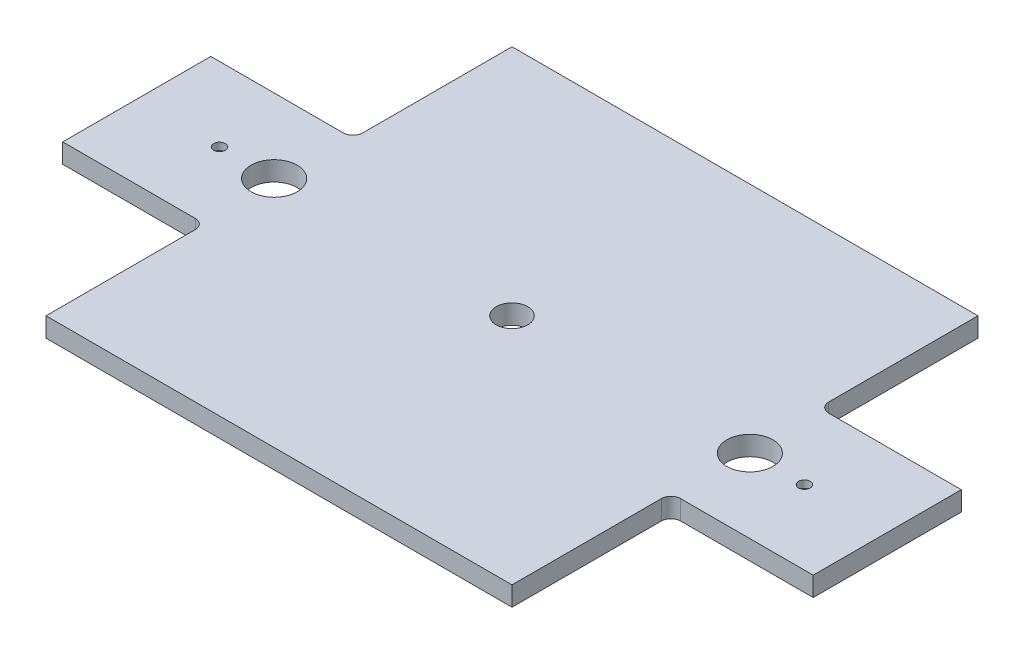
SolidWorks part; units mm, degrees
ref_plane "前视基准面" through (0, 0, 0) normal (0, 0, 1) x (1, 0, 0)
ref_plane "上视基准面" through (0, 0, 0) normal (0, 1, 0) x (1, 0, 0)
ref_plane "右视基准面" through (0, 0, 0) normal (1, 0, 0) x (0, 0, -1)
sketch "草图1" plane through (0, 0, 0) normal (0, 1, 0) x (1, 0, 0)
  line L0 (-480, 480) -> (480, 480)
  line L1 (480, 480) -> (480, 152.5)
  line L2 (480, 152.5) -> (773, 152.5)
  line L3 (773, 152.5) -> (773, -152.5)
  line L4 (773, -152.5) -> (480, -152.5)
  line L5 (480, -152.5) -> (480, -480)
  line L6 (480, -480) -> (-480, -480)
  line L7 (-480, -480) -> (-480, -152.5)
  line L8 (-480, -152.5) -> (-773, -152.5)
  line L9 (-773, -152.5) -> (-773, 152.5)
  line L10 (-773, 152.5) -> (-480, 152.5)
  line L11 (-480, 152.5) -> (-480, 480)
  line L12 (480, 480) -> (-480, -480) construction
  point P3 (0, 480)
  point P10 (0, 0)
  dimension "D1" = 960
  dimension "D2" = 960
  dimension "D3" = 305
  dimension "D4" = 293
extrude "凸台-拉伸1" add sketch "草图1" along normal blind 40
sketch "草图2" plane through (0, 0, 0) normal (0, -1, 0) x (1, 0, 0)
  line L0 (-773, -152.5) -> (-773, 152.5) construction
  line L1 (-773, 152.5) -> (-480, 152.5) construction
  circle A0 centre (602.5, 0) radius 20
  dimension "D1" = 40
  dimension "D2" = 1375.5
  dimension "D3" = 152.5
extrude "切除-拉伸1" cut sketch "草图2" against normal blind 10
hole_wizard "打孔尺寸(%根据)内六角圆柱头螺钉的类型0" positions "草图3" profile "草图4" counterbore size "M14" standard "GB" end condition through all
sketch "草图3" plane through (0, 40, 0) normal (0, 1, 0) x (1, 0, 0)
  line L0 (-480, -152.5) -> (-480, -480) construction
  line L1 (-480, -480) -> (480, -480) construction
  point P0 (602.5, 0)
  dimension "D1" = 1082.5
  dimension "D2" = 480
sketch "草图4" plane through (602.5, 40, 0) normal (1, 0, 0) x (0, 0, 1)
  line L0 (0, 0) -> (0, 40)
  line L1 (0, 40) -> (7.75, 40)
  line L3 (7.75, 40) -> (7.75, 15)
  line L4 (7.75, 15) -> (12, 15)
  line L5 (12, 15) -> (12, 0)
  line L7 (12, 0) -> (0, 0)
  line L11 (0, -6.35) -> (0, 107.95) construction
  dimension "通孔孔直径" = 15.5
  dimension "通孔孔深度" = 40
  dimension "柱形沉头孔直径" = 24
  dimension "柱形沉头孔深度" = 15
mirror "镜向1" about plane through (0, 0, 0) normal (1, 0, 0) of "切除-拉伸1", "打孔尺寸(%根据)内六角圆柱头螺钉的类型0"
sketch "草图5" plane through (0, 0, 0) normal (0, -1, 0) x (1, 0, 0)
  line L0 (-773, -152.5) -> (-773, 152.5) construction
  line L1 (-773, 152.5) -> (-480, 152.5) construction
  circle A0 centre (490, 0) radius 47.5
  dimension "D1" = 95
  dimension "D2" = 1263
  dimension "D3" = 152.5
extrude "切除-拉伸2" cut sketch "草图5" against normal through all
mirror "镜向2" about plane through (0, 0, 0) normal (1, 0, 0) of "切除-拉伸2"
sketch "草图6" plane through (0, 40, 0) normal (0, 1, 0) x (1, 0, 0)
  line L0 (-480, -152.5) -> (-480, -480) construction
  line L1 (-480, -480) -> (480, -480) construction
  circle A0 centre (0, 0) radius 32.5
  dimension "D1" = 65
  dimension "D2" = 480
  dimension "D3" = 480
extrude "切除-拉伸3" cut sketch "草图6" against normal through all
fillet "圆角1" radius 20 4 edges at (-480, 20, 152.5) (-480, 20, -152.5) (480, 20, 152.5) (480, 20, -152.5)
